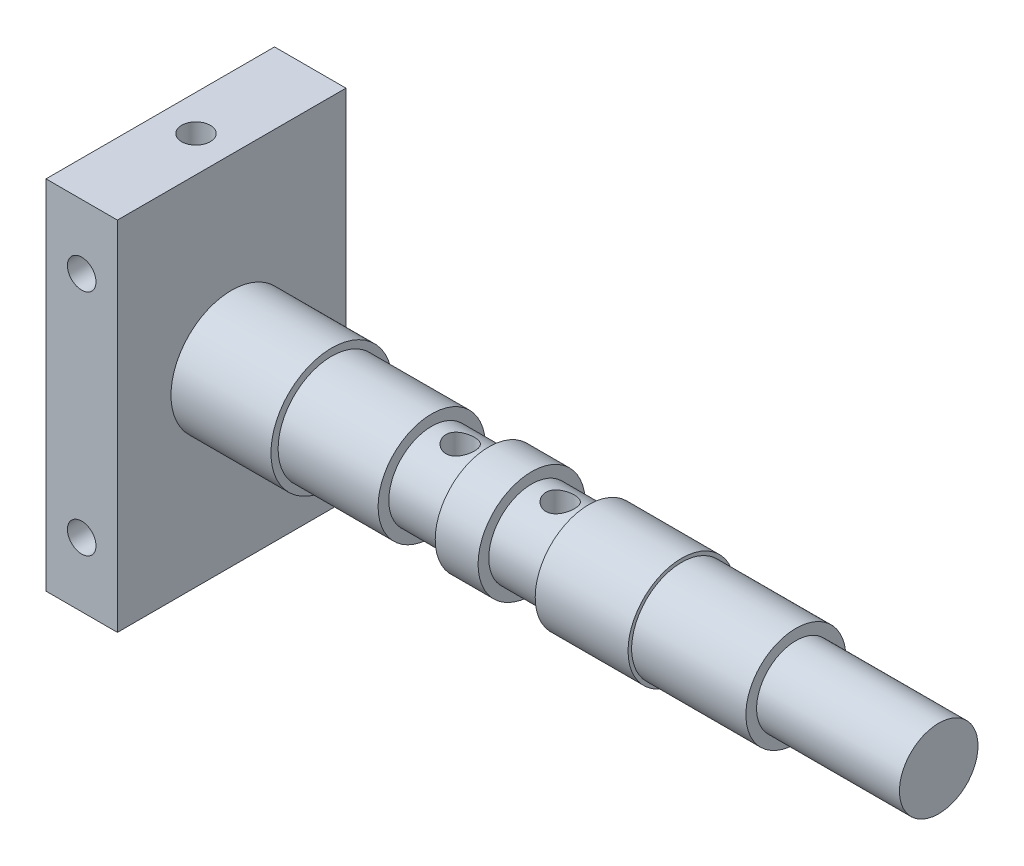
from build123d import *

# Parameters (mm, degrees)
SKETCH1_W           = 32
SKETCH1_H           = 50
BOSS_EXTRUDE1_DEPTH = 10
SKETCH2_R           = 8.5
BOSS_EXTRUDE2_DEPTH = 14
SKETCH3_R           = 2
CUT_EXTRUDE1_DEPTH  = 24
SKETCH4_R           = 2
CUT_EXTRUDE2_DEPTH  = 45
SKETCH5_R           = 7.5
BOSS_EXTRUDE3_DEPTH = 65
SKETCH6_W           = 8
SKETCH6_H           = 1.5
SKETCH7_R           = 5.5
BOSS_EXTRUDE4_DEPTH = 20
SKETCH9_W           = 16
SKETCH9_H           = 0.5
SKETCH10_R          = 2.5
CUT_EXTRUDE3_DEPTH  = 66
SKETCH11_R          = 2
CUT_EXTRUDE4_DEPTH  = 24


with BuildPart() as part:
    # Sketch1 → Boss-Extrude1 (new body)
    with BuildSketch(Plane(origin=(0, 0, 0), x_dir=(0, 0, -1), z_dir=(1, 0, 0))):
        Rectangle(SKETCH1_W, SKETCH1_H)
    extrude(amount=BOSS_EXTRUDE1_DEPTH)

    # Sketch2 → Boss-Extrude2 (add)
    with BuildSketch(Plane(origin=(10, 0, 0), x_dir=(0, 0, -1), z_dir=(1, 0, 0))):
        Circle(SKETCH2_R)
    extrude(amount=BOSS_EXTRUDE2_DEPTH)

    # Sketch3 → Cut-Extrude1 (cut)
    with BuildSketch(Plane.XY.offset(16)):
        with Locations((5, 16)):
            Circle(SKETCH3_R)
        with Locations((5, -16)):
            Circle(SKETCH3_R)
    extrude(amount=-CUT_EXTRUDE1_DEPTH, mode=Mode.SUBTRACT)

    # Sketch4 → Cut-Extrude2 (cut)
    with BuildSketch(Plane(origin=(0, 25, 0), x_dir=(1, 0, 0), z_dir=(0, 1, 0))):
        with Locations(Location((5, 0, 0), (0, 0, 270))):
            Circle(SKETCH4_R)
    extrude(amount=-CUT_EXTRUDE2_DEPTH, mode=Mode.SUBTRACT)

    # Sketch5 → Boss-Extrude3 (add)
    with BuildSketch(Plane(origin=(24, 0, 0), x_dir=(0, 0, -1), z_dir=(1, 0, 0))):
        Circle(SKETCH5_R)
    extrude(amount=BOSS_EXTRUDE3_DEPTH)

    # Sketch6 → Cut-Revolve1 (revolve, cut)
    with BuildSketch(Plane.XY, mode=Mode.PRIVATE) as cut_revolve1_sk:
        with Locations((42, 6.75)):
            Rectangle(SKETCH6_W, SKETCH6_H)
        with Locations((56, 6.75)):
            Rectangle(SKETCH6_W, SKETCH6_H)
    revolve(cut_revolve1_sk.sketch.rotate(Axis((0, 0, 0), (1, 0, 0)), 90), axis=Axis((0, 0, 0), (1, 0, 0)), mode=Mode.SUBTRACT)

    # Sketch7 → Boss-Extrude4 (add)
    with BuildSketch(Plane(origin=(89, 0, 0), x_dir=(0, 0, -1), z_dir=(1, 0, 0))):
        Circle(SKETCH7_R)
    extrude(amount=BOSS_EXTRUDE4_DEPTH)

    # Sketch9 → Cut-Revolve2 (revolve, cut)
    with BuildSketch(Plane.XY, mode=Mode.PRIVATE) as cut_revolve2_sk:
        with Locations((81, 7.25)):
            Rectangle(SKETCH9_W, SKETCH9_H)
    revolve(cut_revolve2_sk.sketch.rotate(Axis((89, 0, 0), (-1, 0, 0)), 270), axis=Axis((89, 0, 0), (-1, 0, 0)), mode=Mode.SUBTRACT)

    # Sketch10 → Cut-Extrude3 (cut)
    with BuildSketch(Plane.ZY):
        Circle(SKETCH10_R)
    extrude(amount=-CUT_EXTRUDE3_DEPTH, mode=Mode.SUBTRACT)

    # Sketch11 → Cut-Extrude4 (cut)
    with BuildSketch(Plane(origin=(0, 25, 0), x_dir=(1, 0, 0), z_dir=(0, 1, 0))):
        with Locations(Location((42, 0, 0), (0, 0, 270))):
            Circle(SKETCH11_R)
        with Locations(Location((56, 0, 0), (0, 0, 270))):
            Circle(SKETCH11_R)
    extrude(amount=-CUT_EXTRUDE4_DEPTH, mode=Mode.SUBTRACT)


solid = part.part
